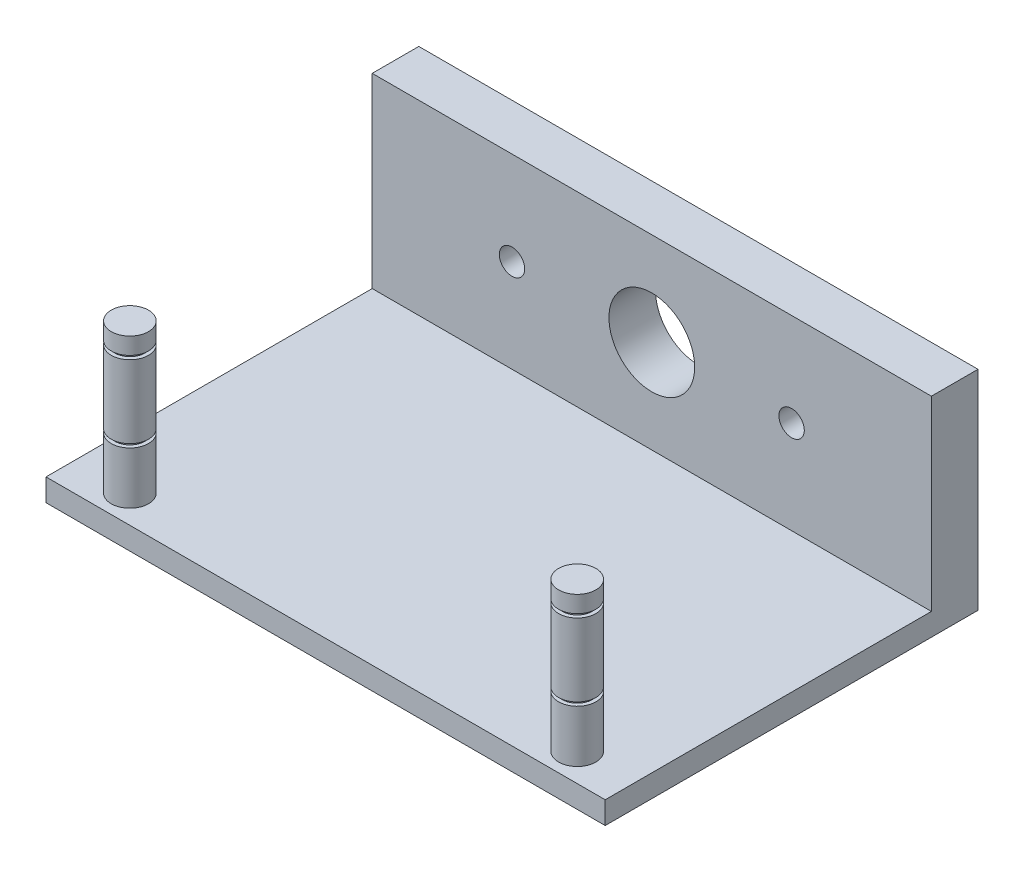
from build123d import *

# Parameters (mm, degrees)
SKETCH1_W                  = 200
SKETCH1_H                  = 50
SKETCH1_R                  = 11.5
BOSS_EXTRUDE1_DEPTH        = 12.5
SKETCH2_W                  = 200
SKETCH2_H                  = 100
BOSS_EXTRUDE2_DEPTH        = 6
M8X1_25_TAPPED_HOLE1_D     = 6.8
M8X1_25_TAPPED_HOLE1_DEPTH = 19.75
M8X1_25_TAPPED_HOLE1_TIP   = 2.042926105
SKETCH6_R                  = 5
BOSS_EXTRUDE3_DEPTH        = 40
SKETCH7_R                  = 7.408343544
SKETCH7_R_2                = 4
SKETCH7_R_3                = 9.473582921
CUT_EXTRUDE1_DEPTH         = 1
SKETCH8_R                  = 11.635219883
SKETCH8_R_2                = 4
SKETCH8_R_3                = 12.853619102
CUT_EXTRUDE2_DEPTH         = 1
CUT_EXTRUDE3_REACH         = 154.105
SKETCH9_W                  = 25
SKETCH9_H                  = 100


with BuildPart() as part:
    # Sketch1 → Boss-Extrude1 (new body)
    with BuildSketch(Plane.XY):
        Rectangle(SKETCH1_W, SKETCH1_H)
        Circle(SKETCH1_R, mode=Mode.SUBTRACT)
    extrude(amount=BOSS_EXTRUDE1_DEPTH)

    # Sketch2 → Boss-Extrude2 (add)
    with BuildSketch(Plane.XZ.offset(25)):
        with Locations((0, 50)):
            Rectangle(SKETCH2_W, SKETCH2_H)
    extrude(amount=BOSS_EXTRUDE2_DEPTH)

    # M8x1.25 Tapped Hole1
    with Locations(Plane(origin=(37.5, 0, 0), x_dir=(-1, 0, 0), z_dir=(0, 0, -1))):
        with Locations((0, 0), (75, 0)):
            Hole(M8X1_25_TAPPED_HOLE1_D / 2, depth=M8X1_25_TAPPED_HOLE1_DEPTH)
            with Locations((0, 0, -(M8X1_25_TAPPED_HOLE1_DEPTH + M8X1_25_TAPPED_HOLE1_TIP / 2))):  # 118° drill point
                Cone(0, M8X1_25_TAPPED_HOLE1_D / 2, M8X1_25_TAPPED_HOLE1_TIP, mode=Mode.SUBTRACT)

    # Sketch6 → Boss-Extrude3 (add)
    with BuildSketch(Plane(origin=(0, -25, 0), x_dir=(1, 0, 0), z_dir=(0, 1, 0))):
        with Locations(Location((60, -92.5, 0), (0, 0, 270))):
            Circle(SKETCH6_R)
        with Locations(Location((-60, -92.5, 0), (0, 0, 270))):
            Circle(SKETCH6_R)
    extrude(amount=BOSS_EXTRUDE3_DEPTH)

    # Sketch7 → Cut-Extrude1 (cut)
    # profile 1 of 2: a face of its own
    with BuildSketch(Plane(origin=(0, 10.5, 0), x_dir=(1, 0, 0), z_dir=(0, 1, 0))):
        with Locations((60, -92.5)):
            Circle(SKETCH7_R)
        with Locations(Location((60, -92.5, 0), (0, 0, 270))):
            Circle(SKETCH7_R_2, mode=Mode.SUBTRACT)
    # profile 2 of 2: a face of its own
    with BuildSketch(Plane(origin=(0, 10.5, 0), x_dir=(1, 0, 0), z_dir=(0, 1, 0))):
        with Locations((-60, -92.5)):
            Circle(SKETCH7_R_3)
        with Locations(Location((-60, -92.5, 0), (0, 0, 270))):
            Circle(SKETCH7_R_2, mode=Mode.SUBTRACT)
    extrude(amount=-CUT_EXTRUDE1_DEPTH, mode=Mode.SUBTRACT)

    # Sketch8 → Cut-Extrude2 (cut)
    # profile 1 of 2: a face of its own
    with BuildSketch(Plane(origin=(0, -10, 0), x_dir=(1, 0, 0), z_dir=(0, 1, 0))):
        with Locations((60, -92.5)):
            Circle(SKETCH8_R)
        with Locations(Location((60, -92.5, 0), (0, 0, 270))):
            Circle(SKETCH8_R_2, mode=Mode.SUBTRACT)
    # profile 2 of 2: a face of its own
    with BuildSketch(Plane(origin=(0, -10, 0), x_dir=(1, 0, 0), z_dir=(0, 1, 0))):
        with Locations((-60, -92.5)):
            Circle(SKETCH8_R_3)
        with Locations(Location((-60, -92.5, 0), (0, 0, 270))):
            Circle(SKETCH8_R_2, mode=Mode.SUBTRACT)
    extrude(amount=-CUT_EXTRUDE2_DEPTH, mode=Mode.SUBTRACT)

    # Sketch9 → Cut-Extrude3 (cut, up to next)
    with BuildSketch(Plane.XZ.offset(31), mode=Mode.PRIVATE) as cut_extrude3_sk1:
        with Locations((87.5, 50)):
            Rectangle(SKETCH9_W, SKETCH9_H)
    cut_extrude3_tool1 = extrude(cut_extrude3_sk1.sketch, amount=-CUT_EXTRUDE3_REACH, mode=Mode.PRIVATE) & part.part
    # Sketch9 → Cut-Extrude3 (cut, up to next)
    with BuildSketch(Plane.XZ.offset(31), mode=Mode.PRIVATE) as cut_extrude3_sk2:
        with Locations((-87.5, 50)):
            Rectangle(SKETCH9_W, SKETCH9_H)
    cut_extrude3_tool2 = extrude(cut_extrude3_sk2.sketch, amount=-CUT_EXTRUDE3_REACH, mode=Mode.PRIVATE) & part.part
    add(cut_extrude3_tool1.solids().sort_by_distance((87.5, -31, 50))[0], mode=Mode.SUBTRACT)
    add(cut_extrude3_tool2.solids().sort_by_distance((-87.5, -31, 50))[0], mode=Mode.SUBTRACT)


solid = part.part
